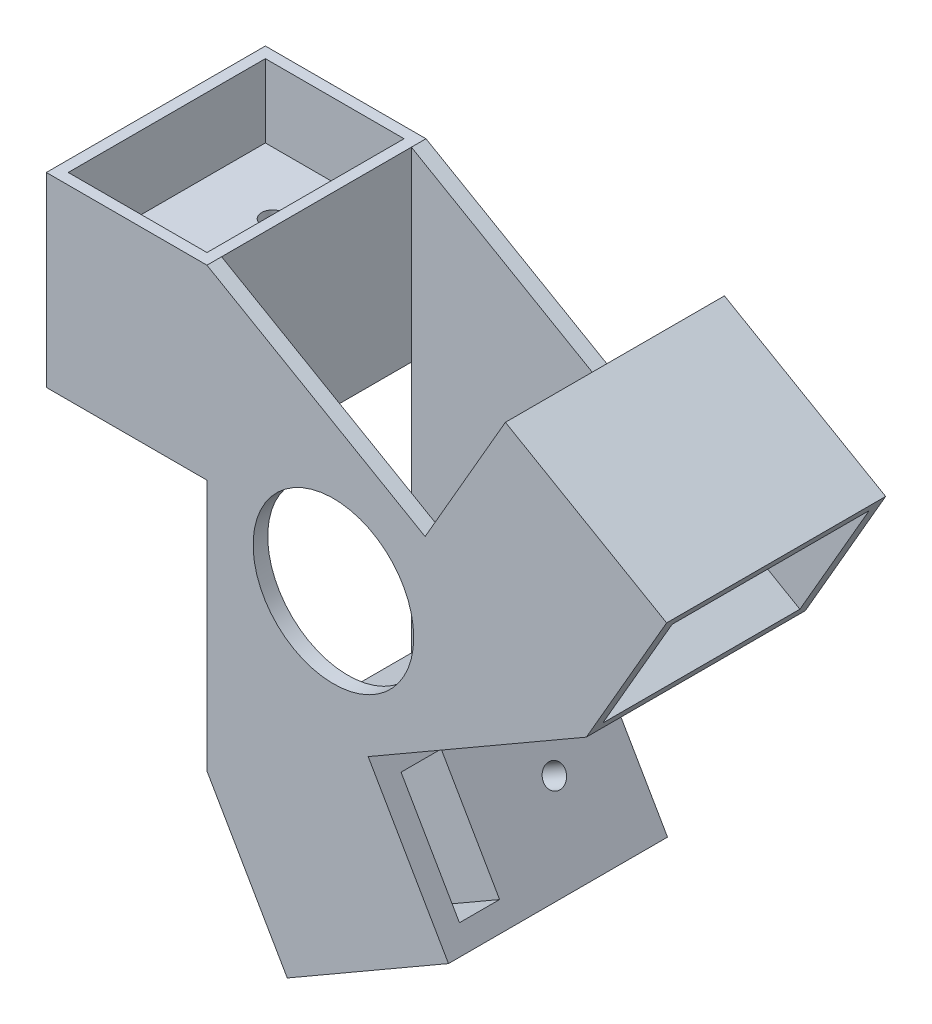
SolidWorks part; units mm, degrees
ref_plane "Front Plane" through (0, 0, 0) normal (0, 0, 1) x (1, 0, 0)
ref_plane "Top Plane" through (0, 0, 0) normal (0, 1, 0) x (1, 0, 0)
ref_plane "Right Plane" through (0, 0, 0) normal (1, 0, 0) x (0, 0, -1)
sketch "Sketch1" plane through (0, 0, 0) normal (0, 0, 1) x (1, 0, 0)
  line L0 (0, 0) -> (0, 345)
  line L1 (0, 600) -> (298.7788, 427.5)
  line L2 (519.6152, 300) -> (220.8365, 127.5)
  line L3 (219.3931, 300) -> (417.4044, 300) construction
  line L4 (219.3931, 300) -> (235.5476, 327.9804) construction
  line L6 (0, 345) -> (-220, 345)
  line L7 (-220, 345) -> (-220, 600)
  line L8 (-220, 600) -> (0, 600)
  line L9 (298.7788, 427.5) -> (408.7788, 618.0256)
  line L10 (408.7788, 618.0256) -> (629.6152, 490.5256)
  line L11 (629.6152, 490.5256) -> (519.6152, 300)
  line L12 (220.8365, 127.5) -> (330.8365, -63.0256)
  line L13 (330.8365, -63.0256) -> (110, -190.5256)
  line L14 (110, -190.5256) -> (0, 0)
  point P24 (173.2051, 300)
  dimension "D3" = 600
  dimension "D5" = 45
  dimension "D6" = 3
  dimension "D7" = 220
extrude "Boss-Extrude1" add sketch "Sketch1" along normal blind 300
sketch "Sketch2" plane through (0, 0, 0) normal (0, 0, -1) x (-1, 0, 0)
  line L0 (0, 600) -> (0, 0)
  line L1 (0, 0) -> (-519.6152, 300)
  line L2 (-519.6152, 300) -> (0, 600)
  line L3 (-298.7788, 427.5) -> (0, 600) construction
  line L4 (-220.8365, 127.5) -> (-519.6152, 300) construction
  line L5 (0, 345) -> (0, 0) construction
  dimension "D1" = 0
  dimension "D2" = 0
  dimension "D3" = 0
extrude "Cut-Extrude2" cut sketch "Sketch2" against normal blind 260 from offset 20 offset against normal yes
sketch "Sketch3" plane through (0, 0, 0) normal (0, 0, -1) x (-1, 0, 0)
  line L0 (0, 600) -> (0, 0) construction
  line L1 (0, 0) -> (-519.6152, 300) construction
  line L2 (-519.6152, 300) -> (0, 600) construction
  line L4 (-259.8076, 150) -> (0, 600) construction
  line L5 (0, 300) -> (-519.6152, 300) construction
  circle A0 centre (-173.2051, 300) radius 25
  dimension "D1" = 50
extrude "Cut-Extrude3" cut sketch "Sketch3" against normal through all
sketch "Sketch4" plane through (0, 0, 0) normal (-0.866, -0.5, 0) x (0, 0, 1)
  line L0 (300, 0) -> (300, -220) construction
  line L1 (300, -220) -> (0, -220) construction
  line L2 (270, -30) -> (215, -30)
  line L3 (270, -30) -> (270, -190)
  line L4 (270, -190) -> (215, -190)
  line L5 (215, -30) -> (215, -190)
  line L6 (280, 0) -> (20, 0) construction
  circle A0 centre (100, -110) radius 15
  dimension "D1" = 30
  dimension "D2" = 200
  dimension "D3" = 30
  dimension "D4" = 30
  dimension "D5" = 30
  dimension "D6" = 55
extrude "Cut-Extrude4" cut sketch "Sketch4" against normal through all
sketch "Sketch5" plane through (0, 600, 0) normal (0, 1, 0) x (1, 0, 0)
  line L0 (0, -300) -> (-220, -300) construction
  line L1 (-220, -300) -> (-220, 0) construction
  line L2 (-30, -270) -> (-190, -270)
  line L3 (-30, -270) -> (-30, -215)
  line L4 (-30, -215) -> (-190, -215)
  line L5 (-190, -270) -> (-190, -215)
  line L6 (0, -280) -> (0, -20) construction
  circle A0 centre (-110, -100) radius 15
  dimension "D1" = 30
  dimension "D2" = 200
  dimension "D3" = 55
  dimension "D4" = 30
  dimension "D5" = 30
  dimension "D6" = 30
extrude "Cut-Extrude5" cut sketch "Sketch5" against normal through all
sketch "Sketch7" plane through (259.8076, -150, 0) normal (0.866, -0.5, 0) x (0, 0, -1)
  line L0 (-300, 519.6152) -> (-300, 739.6152) construction
  line L1 (-300, 739.6152) -> (0, 739.6152) construction
  line L2 (-270, 549.6152) -> (-215, 549.6152)
  line L3 (-270, 549.6152) -> (-270, 709.6152)
  line L4 (-270, 709.6152) -> (-215, 709.6152)
  line L5 (-215, 549.6152) -> (-215, 709.6152)
  line L6 (-280, 519.6152) -> (-20, 519.6152) construction
  circle A0 centre (-100, 629.6152) radius 15
  dimension "D1" = 30
  dimension "D2" = 200
  dimension "D3" = 30
  dimension "D4" = 30
  dimension "D5" = 30
  dimension "D6" = 55
extrude "Cut-Extrude6" cut sketch "Sketch7" against normal through all
sketch "Sketch8" plane through (0, 0, 300) normal (0, 0, 1) x (1, 0, 0)
  circle A0 centre (173.2051, 300) radius 110
  dimension "D1" = 220
extrude "Cut-Extrude7" cut sketch "Sketch8" against normal up to next
sketch "Sketch9" plane through (0, 0, 0) normal (-0.866, -0.5, 0) x (0, 0, 1)
  line L0 (300, -220) -> (0, -220) construction
  line L1 (285, -15) -> (15, -15)
  line L2 (285, -15) -> (285, -205)
  line L3 (285, -205) -> (15, -205)
  line L4 (15, -15) -> (15, -205)
  line L5 (300, 0) -> (300, -220) construction
  line L6 (280, 0) -> (20, 0) construction
  line L7 (0, 0) -> (0, -220) construction
  dimension "D1" = 15
  dimension "D2" = 15
  dimension "D3" = 15
  dimension "D4" = 15
extrude "Cut-Extrude8" cut sketch "Sketch9" against normal blind 100
pattern_circular "CirPattern1" count 3 over 360 about axis through (173.2051, 300, 0) along (0, 0, 1) of "Cut-Extrude8"
